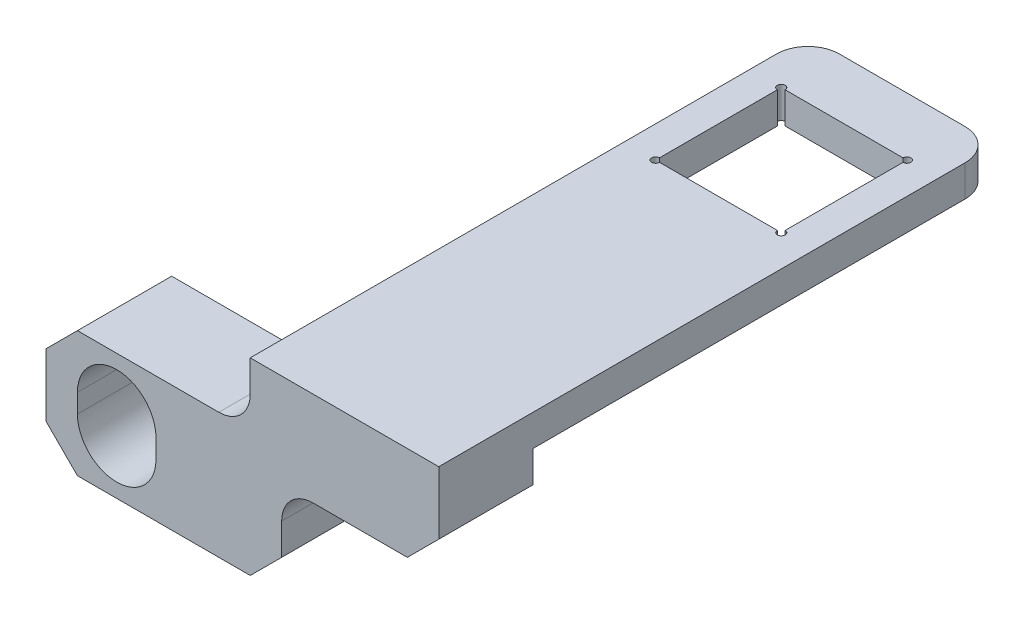
SolidWorks part; units mm, degrees
ref_plane "Front Plane" through (0, 0, 0) normal (0, 0, 1) x (1, 0, 0)
ref_plane "Top Plane" through (0, 0, 0) normal (0, 1, 0) x (1, 0, 0)
ref_plane "Right Plane" through (0, 0, 0) normal (1, 0, 0) x (0, 0, -1)
sketch "Sketch1" plane through (0, 0, 0) normal (0, 1, 0) x (1, 0, 0)
  line L1 (-6, 21.75) -> (6, 21.75)
  line L2 (-6, 21.75) -> (-6, -21.75)
  line L3 (-6, -21.75) -> (6, -21.75)
  line L4 (6, 21.75) -> (6, -21.75)
  line L5 (-6, 21.75) -> (6, -21.75) construction
  line L6 (-6, -21.75) -> (6, 21.75) construction
  point P0 (0, 0)
  dimension "D1" = 12
  dimension "D2" = 43.5
extrude "Boss-Extrude1" add sketch "Sketch1" along normal blind 2
hole_wizard "M3 Tapped Hole1" positions "3DSketch2" profile "Sketch5" tap size "M3" standard "Gb"
sketch3d "3DSketch2"
  point P0 (0, 2, 17.75)
  dimension "D1" = 6
  dimension "D2" = 4
sketch "Sketch5" plane through (0, 2, 17.75) normal (1, 0, 0) x (0, 0, 1)
  line L0 (0, 0) -> (0, 8.2511)
  line L1 (0, 8.2511) -> (1.25, 7.5)
  line L2 (1.25, 7.5) -> (1.25, 0)
  line L5 (1.25, 0) -> (0, 0)
  line L10 (0, 8.2511) -> (-1.25, 7.5) construction
  line L11 (0, -6.35) -> (0, 107.95) construction
  dimension "螺纹孔钻头直径" = 2.5
  dimension "螺纹孔钻头深度" = 7.5
  dimension "导头角度" = 118
cosmetic thread "Cosmetic Thread1" parameters "D1"=2, "D2"=3
sketch "Sketch6" plane through (0, 0, 21.75) normal (0, 0, 1) x (1, 0, 0)
  line L1 (6, 2) -> (-19, 2)
  line L2 (6, 2) -> (6, -10)
  line L3 (6, -10) -> (-19, -10)
  line L4 (-19, 2) -> (-19, -10)
  dimension "D1" = 12
  dimension "D2" = 25
extrude "Boss-Extrude2" add sketch "Sketch6" against normal blind 14
sketch "Sketch7" plane through (0, 2, 0) normal (0, 1, 0) x (1, 0, 0)
  line L0 (-19, -7.75) -> (-19, -21.75) construction
  line L1 (6, -21.75) -> (-19, -21.75)
  line L2 (6, -21.75) -> (6, -13.75)
  line L3 (6, -13.75) -> (-19, -13.75)
  line L4 (-19, -21.75) -> (-19, -13.75)
  dimension "D1" = 8
extrude "Cut-Extrude4" cut sketch "Sketch7" against normal through all
sketch "Sketch8" plane through (0, 0, 13.75) normal (0, 0, 1) x (1, 0, 0)
  line L0 (6, -10) -> (-19, -10) construction
  line L1 (6, -10) -> (6, 2) construction
  circle A0 centre (-14.5, -6) radius 2.5
  dimension "D2" = 5
  dimension "D3" = 20.5
  dimension "D1" = 4
extrude "Cut-Extrude5" cut sketch "Sketch8" against normal blind 15
sketch "Sketch9" plane through (0, 0, 13.75) normal (0, 0, 1) x (1, 0, 0)
  line L0 (-19, -10) -> (-19, 2) construction
  line L1 (-6, 2) -> (-19, 2)
  line L2 (-6, 2) -> (-6, -2)
  line L3 (-6, -2) -> (-19, -2)
  line L4 (-19, 2) -> (-19, -2)
  line L5 (6, -10) -> (-19, -10) construction
  line L7 (6, -10) -> (-4, -10)
  line L8 (6, -10) -> (6, -4)
  line L9 (6, -4) -> (-4, -4)
  line L10 (-4, -10) -> (-4, -4)
  dimension "D1" = 8
  dimension "D2" = 6
  dimension "D3" = 10
extrude "Cut-Extrude6" cut sketch "Sketch9" against normal blind 18
chamfer "Chamfer2" distance 2 angle 45 4 edges at (-4, -10, 10.75) (-19, -10, 10.75) (-19, -2, 10.75) (6, -4, 10.75)
fillet "Fillet1" radius 2 2 edges at (-4, -4, 10.75) (-6, -2, 10.75)
fillet "Fillet2" radius 2 2 edges at (6, 1, -21.75) (-6, 1, -21.75)
sketch "Sketch3" plane through (0, 2, 0) normal (0, 1, 0) x (1, 0, 0)
  line L0 (0, 0) -> (0, 50000) construction
  line L1 (6, -13.75) -> (-6, -13.75) construction
  line L2 (-4, 10.05) -> (4, 10.05)
  line L3 (-4, 10.05) -> (-4, 18.05)
  line L4 (-4, 18.05) -> (4, 18.05)
  line L5 (4, 10.05) -> (4, 18.05)
  line L6 (-4, 10.05) -> (4, 18.05) construction
  line L7 (-4, 18.05) -> (4, 10.05) construction
  point P3 (0, 14.05)
  dimension "D1" = 27.8
  dimension "D2" = 8
  dimension "D3" = 8
extrude "Cut-Extrude2" cut sketch "Sketch3" against normal blind 10
sketch "Sketch10" plane through (0, 2, 0) normal (0, 1, 0) x (1, 0, 0)
  circle A0 centre (-4, 10.05) radius 0.25
  circle A1 centre (4, 10.05) radius 0.25
  circle A2 centre (-4, 18.05) radius 0.25
  circle A3 centre (4, 18.05) radius 0.25
  dimension "D1" = 0.5
extrude "Cut-Extrude7" cut sketch "Sketch10" against normal blind 10
sketch "Sketch11" plane through (0, 0, 13.75) normal (0, 0, 1) x (1, 0, 0)
  line L0 (-14.5, -5.4) -> (-14.5, -6.6) construction
  line L1 (-12, -5.4) -> (-12, -6.6)
  line L2 (-17, -5.4) -> (-17, -6.6)
  arc A0 (-12, -5.4) -> (-17, -5.4) centre (-14.5, -5.4) ccw
  arc A1 (-17, -6.6) -> (-12, -6.6) centre (-14.5, -6.6) ccw
  circle A2 centre (-14.5, -6) radius 2.5 construction
  point P2 (-14.5, -6)
  dimension "D1" = 1.2
extrude "Cut-Extrude8" cut sketch "Sketch11" against normal blind 10
